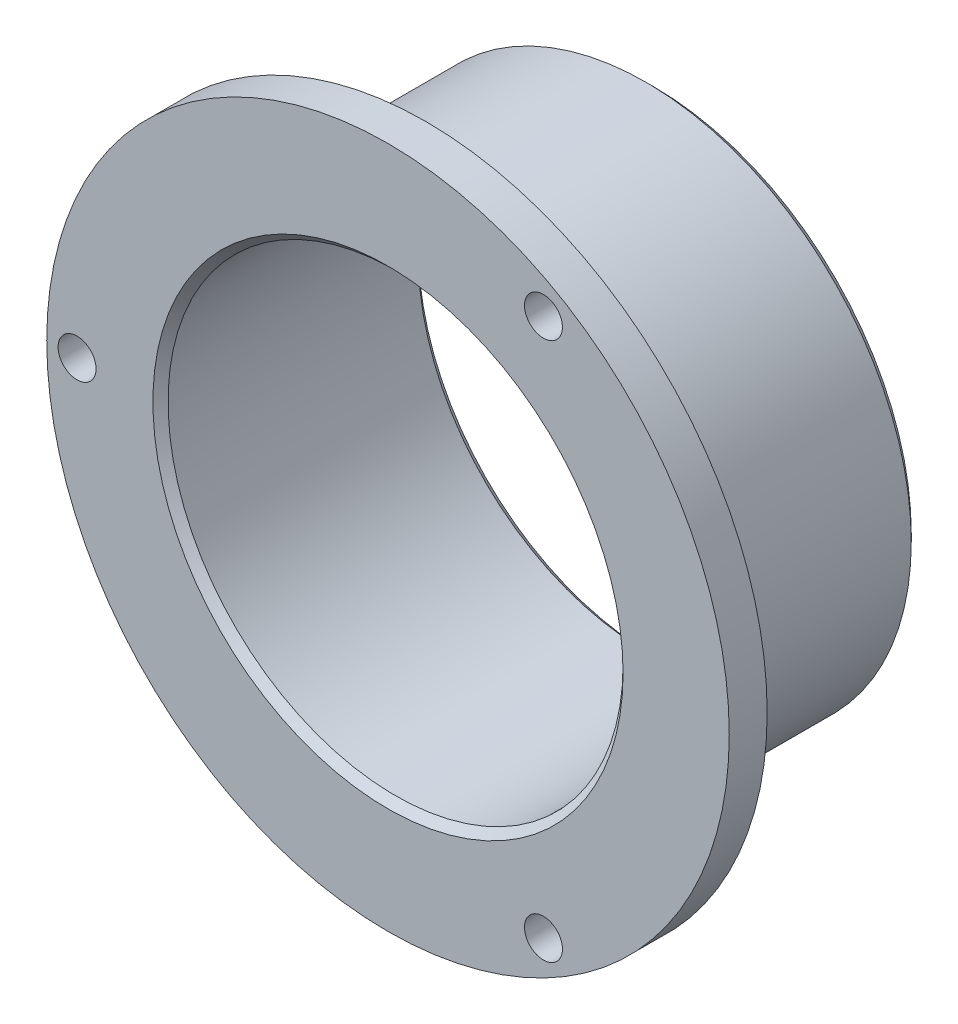
SolidWorks part; units mm, degrees
ref_plane "Front Plane" through (0, 0, 0) normal (0, 0, 1) x (1, 0, 0)
ref_plane "Top Plane" through (0, 0, 0) normal (0, 1, 0) x (1, 0, 0)
ref_plane "Right Plane" through (0, 0, 0) normal (1, 0, 0) x (0, 0, -1)
sketch "Sketch1" plane through (0, 0, 0) normal (0, 0, 1) x (1, 0, 0)
  circle A0 centre (0, 0) radius 35
  circle A1 centre (0, 0) radius 30
  dimension "D1" = 70
  dimension "D2" = 60
extrude "Boss-Extrude1" add sketch "Sketch1" along normal blind 30
sketch "Sketch2" plane through (0, 0, 30) normal (0, 0, 1) x (1, 0, 0)
  circle A0 centre (0, 0) radius 45
  circle A1 centre (0, 0) radius 30
  dimension "D1" = 90
extrude "Boss-Extrude2" add sketch "Sketch2" along normal blind 5
sketch "Sketch3" plane through (0, 0, 30) normal (0, 0, -1) x (-1, 0, 0)
  circle A0 centre (0, 0) radius 41 construction
  circle A1 centre (41, 0) radius 2.5
  circle A2 centre (-20.5, -35.507) radius 2.5
  circle A3 centre (-20.5, 35.507) radius 2.5
  point P11 (0, 0)
  dimension "D1" = 82
  dimension "D2" = 5
extrude "Cut-Extrude1" cut sketch "Sketch3" against normal blind 50
chamfer "Chamfer1" distance 1 angle 45 3 edges at (30, 0, 0) (35, 0, 0) (30, 0, 35)
